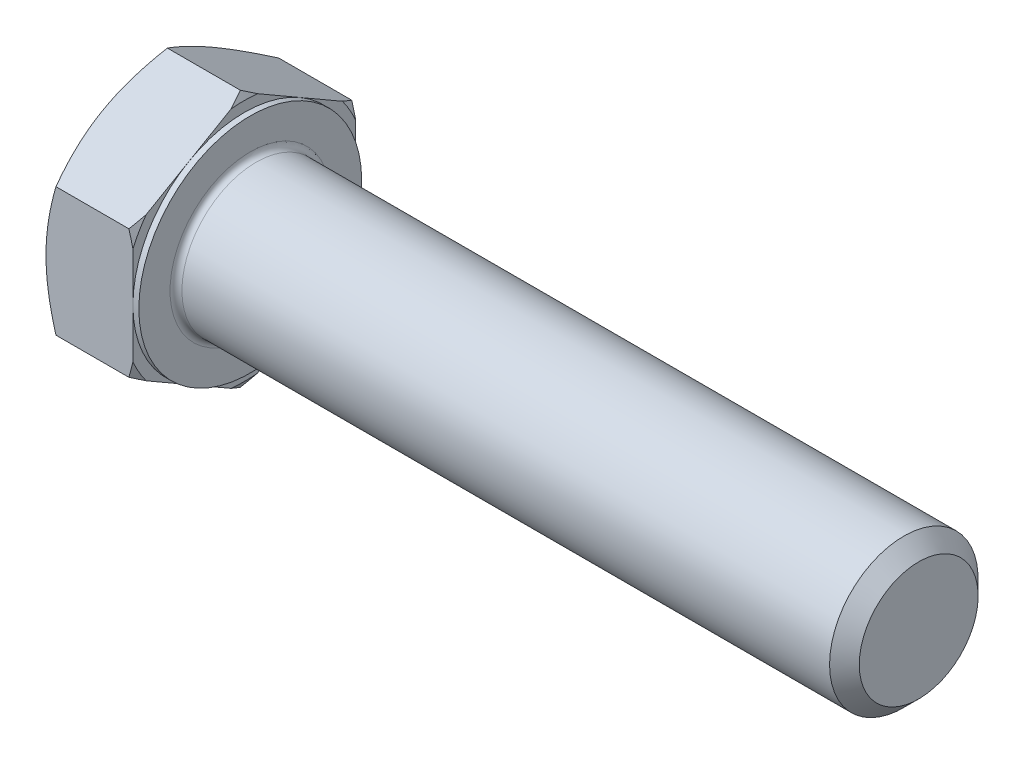
SolidWorks part; units mm, degrees
extrude "基体-拉伸" add sketch "草图1" along normal blind 12.5
sketch "草图1" plane through (0, 0, 0) normal (1, 0, 0) x (0, 0, -1)
  line L0 (15, 8.6603) -> (15, -8.6603)
  line L1 (-15, 8.6603) -> (-15, -8.6603)
  line L2 (15, -8.6603) -> (0, -17.3205)
  line L3 (0, -17.3205) -> (-15, -8.6603)
  line L4 (15, 8.6603) -> (0, 17.3205)
  line L5 (0, 17.3205) -> (-15, 8.6603)
revolve "切除-旋转1" cut sketch "草图3" angle 360 about L6
sketch "草图3" plane through (0, 0, 0) normal (0, 0, 1) x (1, 0, 0)
  line L0 (0, 15) -> (4.2265, 22.3205)
  line L1 (0, 17.3205) -> (0, 8.6603) construction
  line L2 (4.2265, 22.3205) -> (4.2265, 27.3205)
  line L3 (4.2265, 27.3205) -> (-10, 27.3205)
  line L4 (-10, 27.3205) -> (-10, 15)
  line L5 (-10, 15) -> (0, 15)
  line L6 (0, 0) -> (99.06, 0) construction
  line L7 (12.5, 17.3205) -> (0, 17.3205) construction
material "5.6级"
ref_plane "前视" through (0, 0, 0) normal (0, 0, 1) x (1, 0, 0)
ref_plane "上视" through (0, 0, 0) normal (0, 1, 0) x (1, 0, 0)
ref_plane "右视" through (0, 0, 0) normal (1, 0, 0) x (0, 0, -1)
sketch "草图2" plane through (0, 0, 0) normal (0, 0, 1) x (1, 0, 0)
  line L0 (0, 8.6603) -> (0, -8.6603) construction
  line L1 (0, 0) -> (102.5, 0)
  line L2 (0, 0) -> (0, 10)
  line L3 (0, 10) -> (7.7917, 10)
  line L4 (102.5, 0) -> (102.5, 7.835)
  line L5 (12.5, 17.3205) -> (12.5, 8.6603) construction
  line L7 (0, 0) -> (96.52, 0) construction
  line L8 (102.5, -7.835) -> (7.7917, -10) construction
  line L9 (0, -10) -> (7.7917, -10) construction
  line L10 (15, 15.24) -> (15, -1.27) construction
  line L11 (56.5, 15.24) -> (56.5, -1.27) construction
  line L12 (12.5, 8.6603) -> (12.5, -8.6603) construction
  line L13 (7.7917, 10) -> (102.5, 10)
  line L14 (102.5, 10) -> (102.5, 7.835)
revolve "凸台-旋转1" add sketch "草图2" angle 360 about L7
cosmetic thread "螺旋线1" parameters "Thread_length"=46, "Thread_minor"=15.67
sketch "草图5" plane through (0, 0, 0) normal (0, 0, 1) x (1, 0, 0)
  line L0 (12.5, 15) -> (8.2735, 22.3205)
  line L1 (12.5, 17.3205) -> (12.5, 8.6603) construction
  line L2 (8.2735, 22.3205) -> (8.2735, 27.3205)
  line L3 (8.2735, 27.3205) -> (18.2735, 27.3205)
  line L4 (18.2735, 27.3205) -> (18.2735, 15)
  line L5 (18.2735, 15) -> (12.5, 15)
  line L7 (12.5, 17.3205) -> (1.3397, 17.3205) construction
  line L8 (0, 0) -> (99.06, 0) construction
  line L9 (0, 0) -> (99.06, 0) construction
revolve "切除-旋转2" cut sketch "草图5" angle 360 about L8
sketch "草图4" plane through (0, 0, 0) normal (0, 0, 1) x (1, 0, 0)
  line L1 (12.5, 17.3205) -> (12.5, 8.6603) construction
  line L2 (12.5, 15) -> (11.7, 15)
  line L3 (12.5, 15) -> (12.5, 27.3205)
  line L4 (12.5, 27.3205) -> (11.7, 27.3205)
  line L5 (0, 0) -> (95.25, 0) construction
  line L6 (0, 0) -> (96.52, 0) construction
  line L7 (11.7, 15) -> (11.7, 27.3205)
  line L8 (11.1603, 17.3205) -> (1.3397, 17.3205) construction
revolve "切除-旋转3" cut sketch "草图4" angle 360 about L5
chamfer "倒角" distance 2 angle 45 1 edges at (102.5, 0, 10)
fillet "圆角" radius 0.8 1 edges at (12.5, 0, -10)
sketch "草图6" plane through (0, 0, 0) normal (0, 0, 1) x (1, 0, 0)
  line L0 (56.5, -7.835) -> (55.25, -10)
  line L1 (56.5, -7.835) -> (57.75, -10)
  line L2 (57.75, -10) -> (57.75, -12.5)
  line L3 (-3.175, 0) -> (5.1513, 0) construction
  line L5 (57.75, -12.5) -> (55.25, -12.5)
  line L6 (55.25, -12.5) -> (55.25, -10)
revolve "切除-旋转4" [suppressed] cut sketch "草图6" angle 360 about L3
pattern_linear "阵列(线性)1" [suppressed]
equation "\"D3@草图1\" = \"s@草图1\" / 2"
equation "\"D4@草图1\" = \"D3@草图1\""
equation "\"D5@草图1\" = \"D4@草图1\""
equation "\"Thread_minor@螺旋线1\" = \"Minor_dia@草图2\""
equation "\"D1@草图3\" = \"s@草图1\" / 2"
equation "\"D1@草图5\" = \"s@草图1\" / 2"
equation "\"Head_ch_ang@草图5\" = \"Head_ch_ang@草图3\""
equation "\"D1@草图4\" = \"s@草图1\""
equation "\"Thread_length@螺旋线1\" = ((sgn( (\"l@草图2\" - \"p@草图2\" ) - \"h@草图2\" )-1)*( (\"l@草图2\" - \"p@草图2\" ) - \"h@草图2\" ))/-2+ \"h@草图2\""
equation "\"Thread_minor@草图6\" = \"Minor_dia@草图2\""
equation "\"Diameter@草图6\" = \"m@草图2\""
equation "\"Overcut@草图6\" = \"m@草图2\" * 1.25"
equation "\"Start@草图6\" = \"k@基体-拉伸\" + \"l@草图2\" - \"Thread_length@螺旋线1\"  '---Non-countersunk---"
equation "\"Num_threads@阵列(线性)1\" = int( \"Thread_length@螺旋线1\" / \"p@草图2\" + 0.999 )  + 1"
equation "\"Advance@阵列(线性)1\" = \"Thread_length@螺旋线1\" /  (\"Num_threads@阵列(线性)1\" - 1) 'relax it"
equation "\"Num_threads@阵列(线性)1\" = \"Num_threads@阵列(线性)1\" - sgn( \"Num_threads@阵列(线性)1\" - 1) '---chamfered tips only---"
equation "\"Minor_dia@草图2\" = \"m@草图2\"-\"p@草图2\" * 1.732"
equation "\"D1@倒角\" = \"p@草图2\"*0.8"
